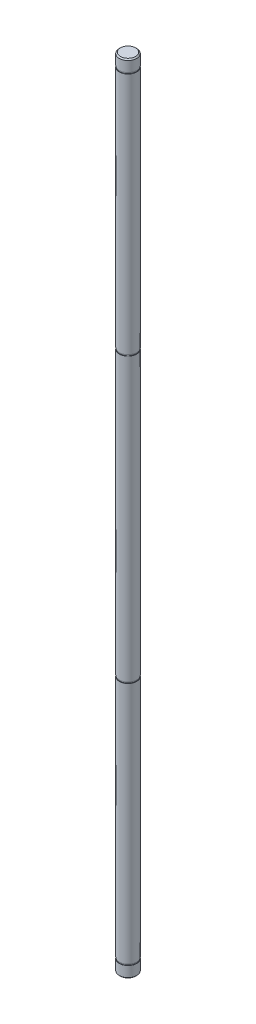
SolidWorks part; units mm, degrees
ref_plane "Front Plane" through (0, 0, 0) normal (0, 0, 1) x (1, 0, 0)
ref_plane "Top Plane" through (0, 0, 0) normal (0, 1, 0) x (1, 0, 0)
ref_plane "Right Plane" through (0, 0, 0) normal (1, 0, 0) x (0, 0, -1)
sketch "Sketch1" plane through (0, 0, 0) normal (0, 1, 0) x (1, 0, 0)
  circle A0 centre (0, 0) radius 7.5
  dimension "D1" = 15
extrude "Boss-Extrude1" add sketch "Sketch1" along normal blind 688
ref_plane "Plane1" through (0, 10, 0) normal (0, -1, 0) x (-1, 0, 0)
sketch "Sketch2" plane through (0, 10, 0) normal (0, -1, 0) x (-1, 0, 0)
  circle A0 centre (0, 0) radius 7.15
  circle A1 centre (0, 0) radius 7.5
  dimension "D1" = 14.3
  dimension "D2" = 15
extrude "Cut-Extrude1" cut sketch "Sketch2" against normal blind 1.1
chamfer "Chamfer1" distance 1 angle 45 2 edges at (0, 688, 7.5) (0, 0, 7.5)
ref_plane "Plane2" through (0, 221, 0) normal (0, -1, 0) x (-1, 0, 0)
sketch "Sketch3" plane through (0, 221, 0) normal (0, -1, 0) x (-1, 0, 0)
  circle A0 centre (0, 0) radius 7.15
  circle A1 centre (0, 0) radius 7.5
  dimension "D1" = 14.3
  dimension "D2" = 15
extrude "Cut-Extrude2" cut sketch "Sketch3" against normal blind 1.1
ref_plane "Plane3" through (0, 344, 0) normal (0, -1, 0) x (-1, 0, 0)
mirror "Mirror1" about plane through (0, 344, 0) normal (0, -1, 0) of "Cut-Extrude1", "Cut-Extrude2"
